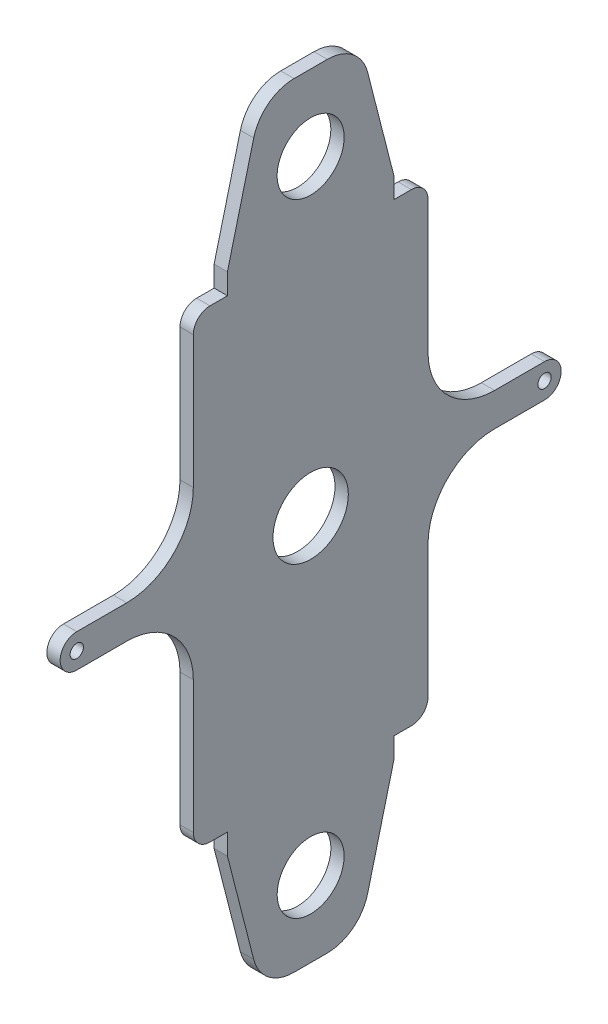
SolidWorks part; units mm, degrees
material "Q235B"
ref_plane "Front Plane" through (0, 0, 0) normal (0, 0, 1) x (1, 0, 0)
ref_plane "Top Plane" through (0, 0, 0) normal (0, 1, 0) x (1, 0, 0)
ref_plane "Right Plane" through (0, 0, 0) normal (1, 0, 0) x (0, 0, -1)
other "Configuration Table"
sketch "Sketch1" plane through (0, 0, 0) normal (1, 0, 0) x (0, 0, -1)
  line L0 (-281, 20) -> (-221, 20)
  line L1 (-141, 100) -> (-141, 279)
  line L2 (-141, 279) -> (-100, 279)
  line L3 (-100, 279) -> (-100, 304)
  line L4 (-100, 304) -> (-68.4406, 427.3897)
  line L5 (-20, 465) -> (20, 465)
  line L7 (0, 159.282) -> (0, 0) construction
  line L9 (100, 304) -> (68.4406, 427.3897)
  line L10 (100, 279) -> (100, 304)
  line L11 (141, 279) -> (100, 279)
  line L12 (141, 100) -> (141, 279)
  line L13 (281, 20) -> (221, 20)
  line L14 (281, -20) -> (221, -20)
  line L15 (141, -100) -> (141, -279)
  line L16 (141, -279) -> (100, -279)
  line L17 (100, -279) -> (100, -304)
  line L18 (100, -304) -> (68.4406, -427.3897)
  line L19 (-20, -465) -> (20, -465)
  line L20 (-100, -304) -> (-68.4406, -427.3897)
  line L21 (-100, -279) -> (-100, -304)
  line L22 (-141, -279) -> (-100, -279)
  line L23 (-141, -100) -> (-141, -279)
  line L24 (-281, -20) -> (-221, -20)
  arc A0 (-281, 20) -> (-281, -20) centre (-281, 0) ccw
  circle A1 centre (0, 374) radius 40.25
  circle A2 centre (0, 0) radius 45.25
  arc A3 (-20, 465) -> (-68.4406, 427.3897) centre (-20, 415) ccw
  arc A4 (-221, 20) -> (-141, 100) centre (-221, 100) ccw
  arc A5 (20, 465) -> (68.4406, 427.3897) centre (20, 415) cw
  arc A6 (221, 20) -> (141, 100) centre (221, 100) cw
  circle A7 centre (0, -374) radius 40.25
  arc A8 (221, -20) -> (141, -100) centre (221, -100) ccw
  arc A9 (20, -465) -> (68.4406, -427.3897) centre (20, -415) ccw
  arc A10 (-20, -465) -> (-68.4406, -427.3897) centre (-20, -415) cw
  arc A11 (-221, -20) -> (-141, -100) centre (-221, -100) cw
  arc A12 (281, -20) -> (281, 20) centre (281, 0) ccw
  circle A13 centre (20, -75) radius 4.25
  circle A14 centre (-20, -75) radius 4.25
  circle A15 centre (-20, 442) radius 3.5
  circle A16 centre (20, 442) radius 3.5
  circle A17 centre (-20, -442) radius 4.25
  circle A18 centre (20, -442) radius 4.25
  circle A19 centre (-281, 0) radius 8
  circle A20 centre (281, 0) radius 8
  point P18 (0, 465)
  dimension "D1" = 40
  dimension "D2" = 80.5
  dimension "D12" = 90.5
  dimension "D13" = 50
  dimension "D16" = 80
  dimension "D21" = 8.5
  dimension "D26" = 7
  dimension "D3" = 281
  dimension "D4" = 0
  dimension "D5" = 465
  dimension "D6" = 279
  dimension "D7" = 100
  dimension "D8" = 141
  dimension "D9" = 25
  dimension "D10" = 91
  dimension "D11" = 0
  dimension "D14" = 20
  dimension "D15" = 0
  dimension "D17" = 75
  dimension "D18" = 75
  dimension "D19" = 40
  dimension "D20" = 20
  dimension "D22" = 20
  dimension "D23" = 40
  dimension "D24" = 68
  dimension "D25" = 68
extrude "Boss-Extrude1" add sketch "Sketch1" along normal blind 16
fillet "Fillet1" radius 20 4 edges at (8, -279, -141) (8, -279, 141) (8, 279, -141) (8, 279, 141)
sketch "Sketch2" plane through (0, 0, 0) normal (-1, 0, 0) x (0, 0, 1)
  circle A1 centre (20, -442) radius 4.25 construction
  circle A2 centre (-20, -442) radius 4.25 construction
  circle A3 centre (20, -75) radius 4.25 construction
  circle A4 centre (-20, -75) radius 4.25 construction
  circle A5 centre (20, 442) radius 3.5 construction
  circle A6 centre (-20, 442) radius 3.5 construction
  circle A7 centre (20, -442) radius 4.25
  circle A8 centre (-20, -442) radius 4.25
  circle A9 centre (20, -75) radius 4.25
  circle A10 centre (-20, -75) radius 4.25
  circle A11 centre (20, 442) radius 3.5
  circle A12 centre (-20, 442) radius 3.5
extrude "Boss-Extrude2" add sketch "Sketch2" against normal up to surface (16 mm away) up to face at (16, 0, 0)
hole_wizard "M10 Tapped Hole1" positions "Sketch3" profile "Sketch4" tap size "M10" standard "GB"
sketch "Sketch3" plane through (0, 0, 0) normal (-1, 0, 0) x (0, 0, 1)
  point P0 (-20, 442)
  point P3 (20, 442)
  point P6 (-20, -75)
  point P9 (20, -75)
  point P12 (-20, -442)
  point P15 (20, -442)
sketch "Sketch4" plane through (0, 442, -20) normal (0, 1, 0) x (0, 0, 1)
  line L0 (0, 0) -> (0, 16)
  line L1 (0, 16) -> (4.25, 16)
  line L2 (4.25, 16) -> (4.25, 0)
  line L5 (4.25, 0) -> (0, 0)
  line L11 (0, -6.35) -> (0, 107.95) construction
  dimension "通孔螺纹孔钻头直径" = 8.5
  dimension "通孔螺纹孔钻头深度" = 16
cosmetic thread "Cosmetic thread1" [suppressed] parameters "D1"=20, "D2"=9.5
cosmetic thread "Cosmetic thread2" [suppressed] parameters "D1"=20, "D2"=9.5
